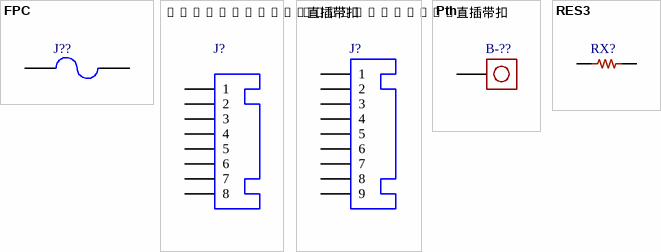
[diagram p0: symbols FPC to RES3]
# Altium schematic symbol library MISC86336.SCHLIB: 5 symbols
Pins are listed as number, name and electrical type; pins without a type are passive.


## FPC
designator J??
footprint 异形电阻
pins: 1, 2

## HX-2.0mm-8P直插带扣
designator J?
HX-2.0mm-8P THT connector with latch
footprint HX2.54-5P直插不带扣 (HX2.54-5P THT connector without latch)
footprint HX2.0-9P
pins: 1, 2, 3, 4, 5, 6, 7, 8

## HX-2.54mm-9P直插带扣
designator J?
HX-2.54mm-9P THT connector with latch
footprint HX2.54-5P直插不带扣 (HX2.54-5P THT connector without latch)
footprint HX2.0-9P
pins: 1, 2, 3, 4, 5, 6, 7, 8, 9

## Pth
designator B-??
Through-hole pad
footprint 4*3 (Through-hole pad)
footprint 35*7*0.3mm
footprint 10*8*0.3mm (Nickel tab)
footprint 30*6*0.5mm
pins: 1

## RES3
designator RX?
Alloy SMD resistor
footprint R1206A (SMD resistor)
footprint R1206L (SMD resistor)
pins: 1, 2